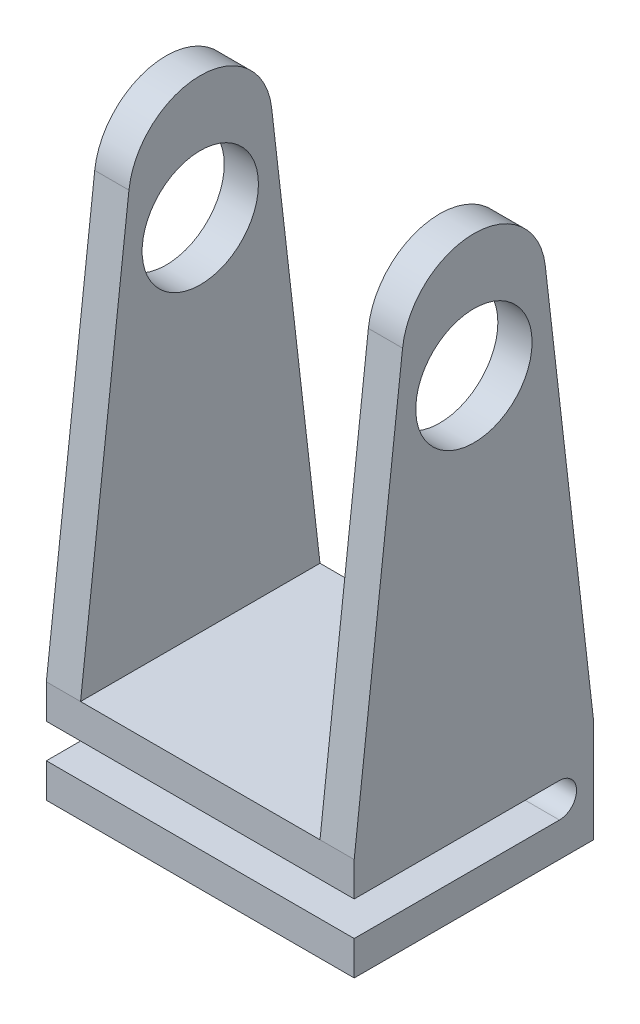
SolidWorks part; units mm, degrees
material "Beech"
ref_plane "Front Plane" through (0, 0, 0) normal (0, 0, 1) x (1, 0, 0)
ref_plane "Top Plane" through (0, 0, 0) normal (0, 1, 0) x (1, 0, 0)
ref_plane "Right Plane" through (0, 0, 0) normal (1, 0, 0) x (0, 0, -1)
sketch "Sketch1" plane through (0, 0, 0) normal (0, 1, 0) x (1, 0, 0)
  line L1 (45, -35) -> (-45, -35)
  line L2 (45, -35) -> (45, 35)
  line L3 (45, 35) -> (-45, 35)
  line L4 (-45, -35) -> (-45, 35)
  line L5 (45, -35) -> (-45, 35) construction
  line L6 (45, 35) -> (-45, -35) construction
  point P0 (0, 0)
  dimension "D1" = 90
  dimension "D2" = 70
extrude "Boss-Extrude1" add sketch "Sketch1" along normal blind 30
sketch "Sketch2" plane through (45, 0, 0) normal (1, 0, 0) x (0, 0, -1)
  line L0 (-20.8613, 152.4095) -> (-35, 30)
  line L1 (20.8613, 152.4095) -> (35, 30)
  line L2 (-35, 30) -> (35, 30) construction
  line L3 (35, 30) -> (-35, 30)
  arc A0 (20.8613, 152.4095) -> (-20.8613, 152.4095) centre (0, 150) ccw
  circle A1 centre (0, 135) radius 17
  dimension "D1" = 42
  dimension "D3" = 34
  dimension "D4" = 105
  dimension "D2" = 150
extrude "Boss-Extrude2" add sketch "Sketch2" against normal blind 10
mirror "Mirror1" about plane through (0, 0, 0) normal (1, 0, 0) of "Boss-Extrude2"
sketch "Sketch3" plane through (45, 0, 0) normal (1, 0, 0) x (0, 0, -1)
  line L0 (-35, 30) -> (-35, 0) construction
  line L1 (-35, 20) -> (25, 20)
  line L2 (-35, 20) -> (-35, 10)
  line L3 (-35, 10) -> (25, 10)
  line L4 (25, 20) -> (25, 10)
  circle A0 centre (25, 15) radius 5
  line M6 (-35, 30) -> (-35, 0)
  dimension "D2" = 10
  dimension "D3" = 15
  dimension "D1" = 60
extrude "Cut-Extrude1" cut sketch "Sketch3" against normal through all contours A0 L1 L3 M6 | L4 A0 | L4 A0
